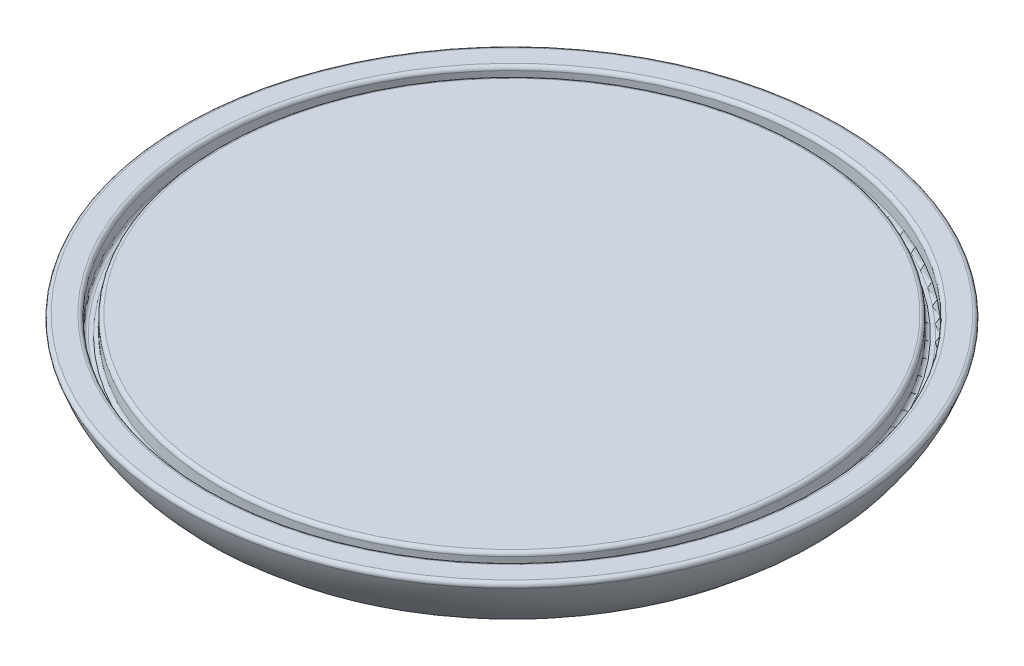
from build123d import *


with BuildPart() as part:
    # Sketch 1 → Revolve1 (revolve)
    with BuildSketch(Plane.XY, mode=Mode.PRIVATE) as revolve1_sk:
        with BuildLine():
            Line((-2, -0.4), (-6.108633541, -0.4))
            ThreePointArc((-6.108633541, -0.4), (-7.8702942, 0.17171836), (-8.960505697, 1.668965517))
            ThreePointArc((-8.960505697, 1.668965517), (-8.946386013, 1.758722022), (-8.865443291, 1.8))
            Line((-8.865443291, 1.8), (-8.35, 1.8))
            ThreePointArc((-8.35, 1.8), (-8.279289322, 1.770710678), (-8.25, 1.7))
            Line((-8.25, 1.7), (-8.25, 1.4))
            ThreePointArc((-8.25, 1.4), (-8.220710678, 1.329289322), (-8.15, 1.3))
            Line((-8.15, 1.3), (-8.05, 1.3))
            ThreePointArc((-8.05, 1.3), (-7.979289322, 1.329289322), (-7.95, 1.4))
            Line((-7.95, 1.4), (-7.95, 1.7))
            ThreePointArc((-7.95, 1.7), (-7.920710678, 1.770710678), (-7.85, 1.8))
            Line((-7.85, 1.8), (0, 1.8))
            Line((0, 1.8), (0, 0.4))
            Line((0, 0.4), (-2, 0.4))
            Line((-2, 0.4), (-2, -0.4))
        make_face()
    revolve(revolve1_sk.sketch.rotate(Axis((0, 0, 0), (0, 1, 0)), 270), axis=Axis((0, 0, 0), (0, 1, 0)))


solid = part.part
